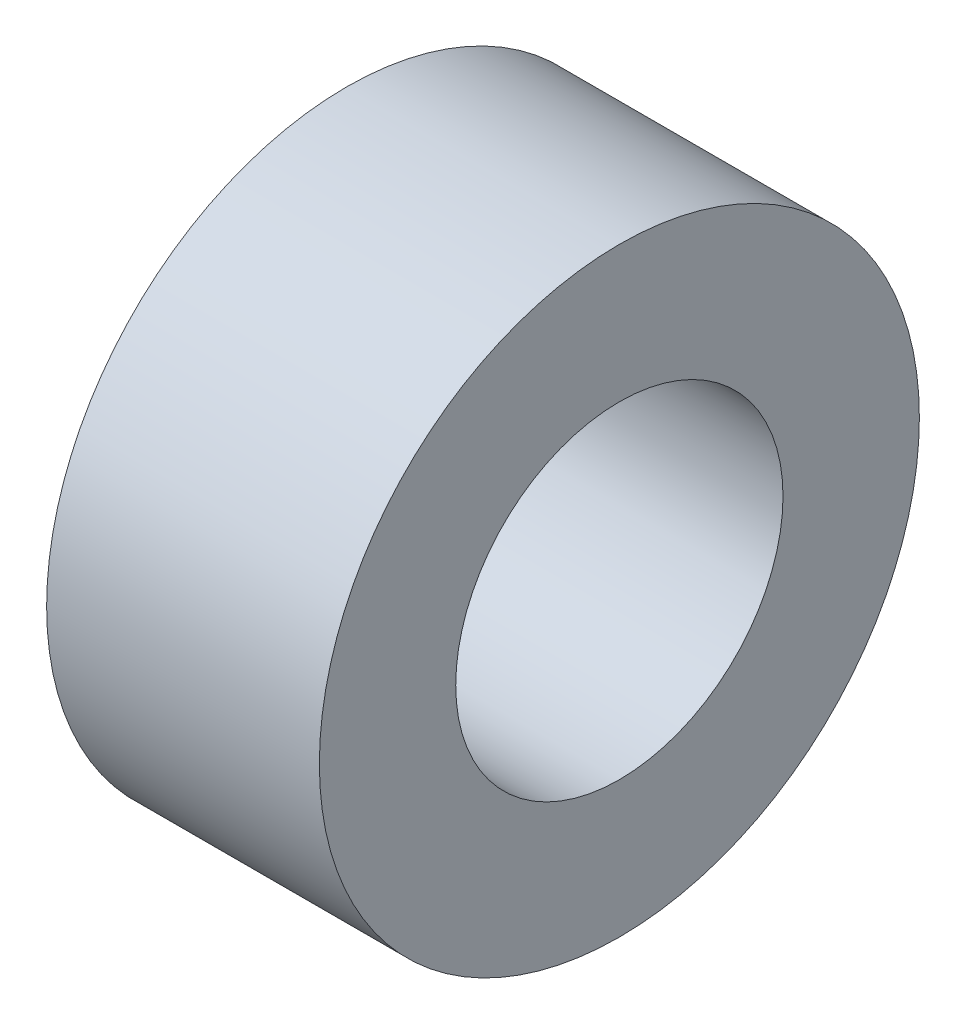
SolidWorks part; units mm, degrees
ref_plane "Front Plane" through (0, 0, 0) normal (0, 0, 1) x (1, 0, 0)
ref_plane "Top Plane" through (0, 0, 0) normal (0, 1, 0) x (1, 0, 0)
ref_plane "Right Plane" through (0, 0, 0) normal (1, 0, 0) x (0, 0, -1)
other "Configuration Table"
sketch "Sketch1" plane through (0, 0, 0) normal (1, 0, 0) x (0, 0, -1)
  circle A0 centre (0, 0) radius 5.5
  circle A1 centre (0, 0) radius 3
  dimension "D1" = 11
  dimension "D2" = 6
extrude "Boss-Extrude1" add sketch "Sketch1" along normal blind 5
